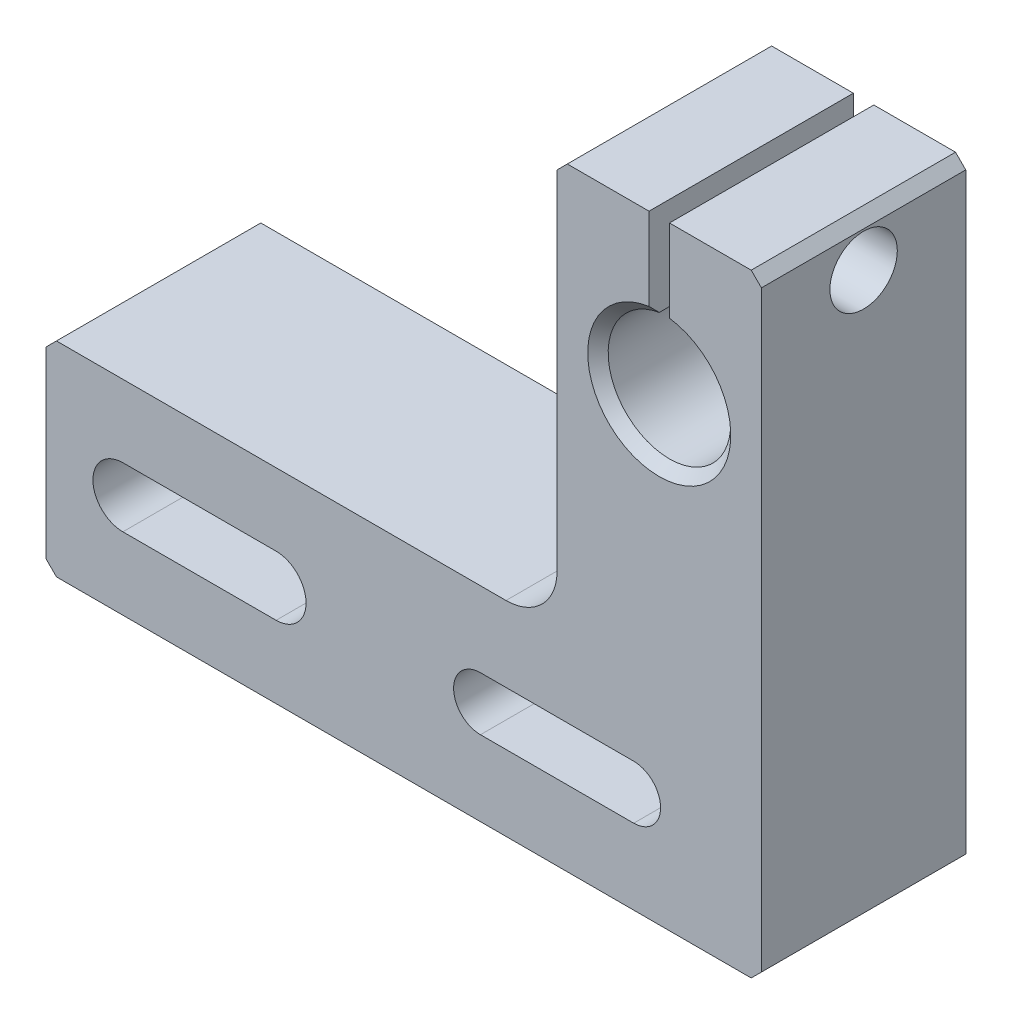
from build123d import *

# Parameters (mm, degrees)
BOSS_EXTRUDE1_DEPTH   = 20
CHAMFER1_SIZE         = 1
M6_TAPPED_HOLE1_D     = 5
M6_TAPPED_HOLE1_DEPTH = 9
M6_TAPPED_HOLE1_TIP   = 1.502151548
HOLE1_D               = 6.6
HOLE1_DEPTH           = 9
CHAMFER2_SIZE         = 1
FILLET1_R             = 5


with BuildPart() as part:
    # Sketch1 → Boss-Extrude1 (new body)
    with BuildSketch(Plane.XY):
        with BuildLine():
            Line((22.049935288, 34.795918367), (22.049935288, -25.204081633))
            Line((22.049935288, -25.204081633), (-47.950064712, -25.204081633))
            Line((-47.950064712, -25.204081633), (-47.950064712, -5.204081633))
            Line((-47.950064712, -5.204081633), (2.049935288, -5.204081633))
            Line((2.049935288, -5.204081633), (2.049935288, 34.795918367))
            Line((2.049935288, 34.795918367), (11.049935288, 34.795918367))
            Line((11.049935288, 34.795918367), (11.049935288, 25.71199815))
            ThreePointArc((11.049935288, 25.71199815), (12.049935288, 13.795918367), (13.049935288, 25.71199815))
            Line((13.049935288, 25.71199815), (13.049935288, 34.795918367))
            Line((13.049935288, 34.795918367), (22.049935288, 34.795918367))
        make_face()
        with BuildLine():
            Line((-40.450064712, -12.275048454), (-25.450064712, -12.275048454))
            ThreePointArc((-25.450064712, -12.275048454), (-22.521031533, -15.204081633), (-25.450064712, -18.133114812))
            Line((-25.450064712, -18.133114812), (-40.450064712, -18.133114812))
            ThreePointArc((-40.450064712, -18.133114812), (-43.379097891, -15.204081633), (-40.450064712, -12.275048454))
        make_face(mode=Mode.SUBTRACT)
        with BuildLine():
            Line((-5.450064712, -12.576085385), (9.549935288, -12.576085385))
            ThreePointArc((9.549935288, -12.576085385), (12.177931536, -15.204081633), (9.549935288, -17.832077881))
            Line((9.549935288, -17.832077881), (-5.450064712, -17.832077881))
            ThreePointArc((-5.450064712, -17.832077881), (-8.07806096, -15.204081633), (-5.450064712, -12.576085385))
        make_face(mode=Mode.SUBTRACT)
    extrude(amount=BOSS_EXTRUDE1_DEPTH)

    # Chamfer1
    chamfer1_edges = [part.edges().sort_by_distance(p)[0] for p in [
        (12.049935288, 13.795918367, 20),
        (12.049935288, 13.795918367, 0),
    ]]
    chamfer(chamfer1_edges, length=CHAMFER1_SIZE)

    # M6 Tapped Hole1
    with Locations(Plane.ZY.offset(-2.049935288)):
        with Locations((10, 30.295918367)):
            Hole(M6_TAPPED_HOLE1_D / 2, depth=M6_TAPPED_HOLE1_DEPTH)
            with Locations((0, 0, -(M6_TAPPED_HOLE1_DEPTH + M6_TAPPED_HOLE1_TIP / 2))):  # 118° drill point
                Cone(0, M6_TAPPED_HOLE1_D / 2, M6_TAPPED_HOLE1_TIP, mode=Mode.SUBTRACT)

    # Hole1
    with Locations(Plane(origin=(22.049935288, 0, 0), x_dir=(0, 0, -1), z_dir=(1, 0, 0))):
        with Locations((-10, 30.295918367)):
            Hole(HOLE1_D / 2, depth=HOLE1_DEPTH)

    # Chamfer2
    chamfer2_edges = [part.edges().sort_by_distance(p)[0] for p in [
        (22.049935288, 34.795918367, 10),
        (22.049935288, -25.204081633, 10),
        (-47.950064712, -25.204081633, 10),
        (-47.950064712, -5.204081633, 10),
        (2.049935288, 34.795918367, 10),
    ]]
    chamfer(chamfer2_edges, length=CHAMFER2_SIZE)

    # Fillet1
    fillet1_edges = [part.edges().sort_by_distance(p)[0] for p in [
        (2.049935288, -5.204081633, 10),
    ]]
    fillet(fillet1_edges, radius=FILLET1_R)


solid = part.part
